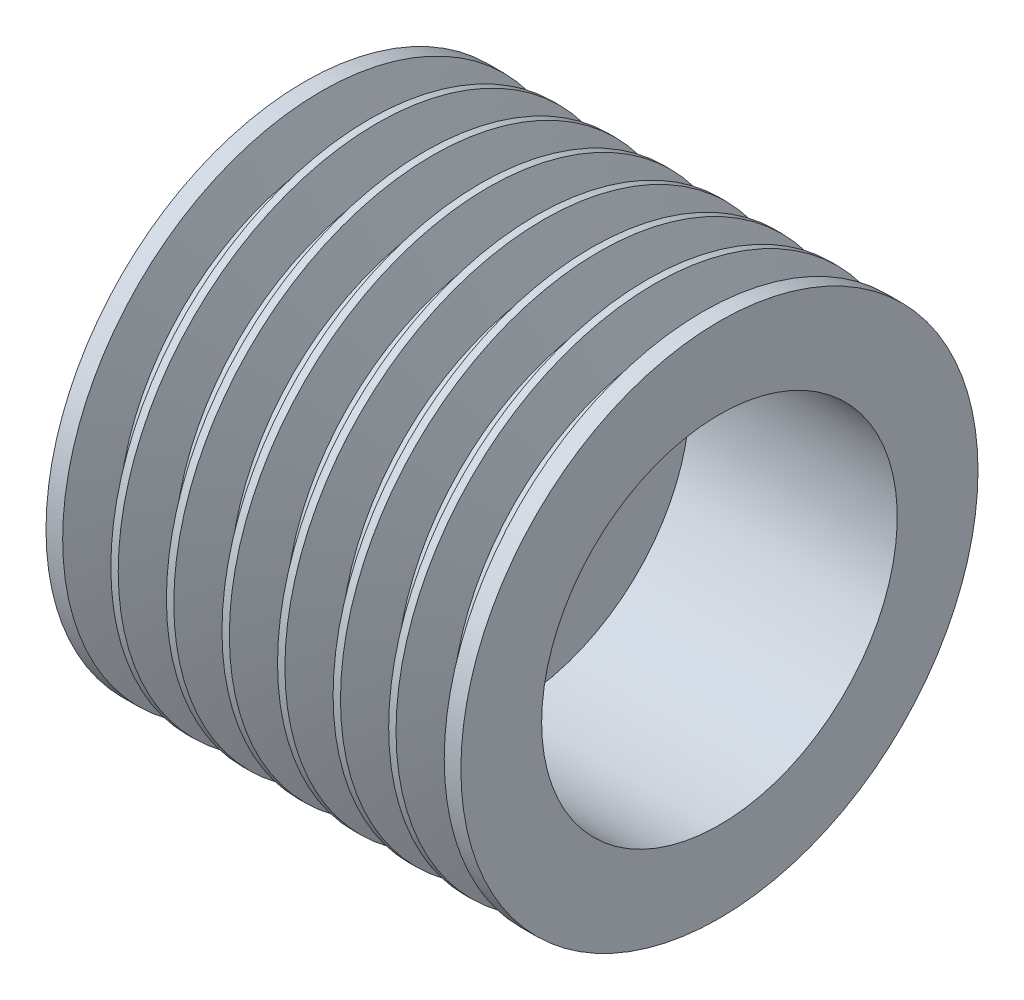
SolidWorks part; units mm, degrees
material "灰铸铁 HT200 "
ref_plane "Front Plane" through (0, 0, 0) normal (0, 0, 1) x (1, 0, 0)
ref_plane "Top Plane" through (0, 0, 0) normal (0, 1, 0) x (1, 0, 0)
ref_plane "Right Plane" through (0, 0, 0) normal (1, 0, 0) x (0, 0, -1)
sketch "Sketch1" plane through (0, 0, 0) normal (0, 0, 1) x (1, 0, 0)
  line L0 (0, 0) -> (218.7952, 0) construction
  line L1 (0, 0) -> (0, 75) construction
  line L2 (0, 37.5) -> (-140, 37.5)
  line L3 (-140, 37.5) -> (-140, 120)
  line L7 (-140, 120) -> (-140, 174.5)
  line L8 (-140, 174.5) -> (140, 174.5)
  line L9 (140, 174.5) -> (140, 120)
  line L10 (140, 120) -> (0, 120)
  line L13 (0, 120) -> (0, 37.5)
  dimension "D1" = 280
  dimension "D2" = 37.5
  dimension "D3" = 120
  dimension "D9" = 174.5
revolve "Revolve1" add sketch "Sketch1" angle 360 about L0
sketch "Sketch2" plane through (0, 0, 0) normal (0, 1, 0) x (1, 0, 0)
  line L0 (0, -238.1643) -> (0, 238.1643) construction
  line L1 (-238.8971, 0) -> (238.8971, 0) construction
  line L2 (-112.5, 198.0555) -> (-112.5, 125.3136) construction
  line L3 (-140, 174.5) -> (-140, -174.5) construction
  line L4 (-131.0801, 181.635) -> (-119.5016, 146)
  line L5 (-119.5016, 146) -> (-105.4984, 146)
  line L6 (-105.4984, 146) -> (-93.9199, 181.635)
  line L7 (-93.9199, 181.635) -> (-131.0801, 181.635)
  line L8 (-136.2383, 166) -> (-90.4467, 166) construction
  line L9 (140, 174.5) -> (-140, 174.5) construction
  point P4 (0, 0)
  point P8 (0, 0)
  point P18 (-126, 166)
  point P19 (-99, 166)
  dimension "D1" = 27.5
  dimension "D2" = 36
  dimension "D3" = 8.5
  dimension "D4" = 27
  dimension "D5" = 28.5
revolve "Cut-Revolve1" cut sketch "Sketch2" angle 360 about L1
sketch "Sketch3" plane through (-140, 0, 0) normal (-1, 0, 0) x (0, 0, 1)
  line L0 (0, 0) -> (0, 53.085) construction
  line L2 (10, -1.3418) -> (-10, -1.3418)
  line L3 (10, -1.3418) -> (10, 42.4)
  line L4 (10, 42.4) -> (-10, 42.4)
  line L5 (-10, -1.3418) -> (-10, 42.4)
  line L6 (10, -1.3418) -> (-10, 42.4) construction
  line L7 (10, 42.4) -> (-10, -1.3418) construction
  circle A2 centre (0, 0) radius 37.5 construction
  point P3 (0, 20.5291)
  dimension "D1" = 20
  dimension "D2" = 79.9
extrude "Cut-Extrude1" cut sketch "Sketch3" against normal through all
pattern_linear "LPattern1" count 7 spacing 37.5 along (1, 0, 0) of "Cut-Revolve1"
